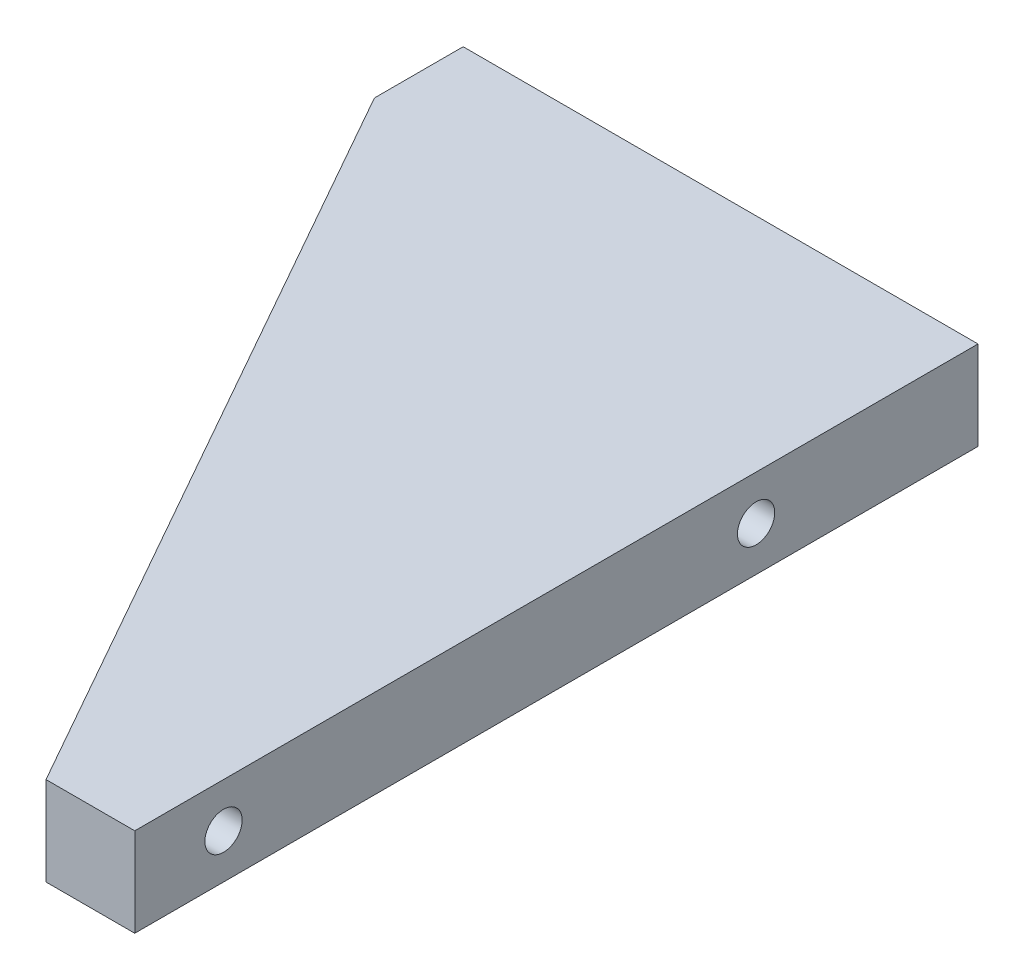
from build123d import *

# Parameters (mm, degrees)
SKETCH_1_W             = 58
SKETCH_1_H             = 95
EXTRUDE_1_DEPTH        = 5
CUT_EXTRUDE_1_DEPTH    = 10
HOLE_WIZARD_M5_1_D     = 4.2
HOLE_WIZARD_M5_1_DEPTH = 12.4
HOLE_WIZARD_M5_1_TIP   = 1.2618073
HOLE_WIZARD_M5_2_D     = 4.2
HOLE_WIZARD_M5_2_DEPTH = 12.4
HOLE_WIZARD_M5_2_TIP   = 1.2618073


with BuildPart() as part:
    # 草图1 → 凸台-拉伸1 (new, symmetric)
    with BuildSketch(Plane(origin=(0, 0, 0), x_dir=(1, 0, 0), z_dir=(0, 1, 0))):
        Rectangle(SKETCH_1_W, SKETCH_1_H)
    extrude(amount=EXTRUDE_1_DEPTH, both=True)

    # 草图2 → 切除-拉伸1 (cut)
    with BuildSketch(Plane(origin=(0, 5, 0), x_dir=(1, 0, 0), z_dir=(0, 1, 0))):
        Polygon((19, -47.5), (-29, 37.5), (-29, -47.5), align=None)
    extrude(amount=-CUT_EXTRUDE_1_DEPTH, mode=Mode.SUBTRACT)

    # M5 螺纹孔1
    with Locations(Plane(origin=(29, 0, 0), x_dir=(0, 0, -1), z_dir=(1, 0, 0))):
        with Locations((-37.5, 0), (22.5, 0)):
            Hole(HOLE_WIZARD_M5_1_D / 2, depth=HOLE_WIZARD_M5_1_DEPTH)
            with Locations((0, 0, -(HOLE_WIZARD_M5_1_DEPTH + HOLE_WIZARD_M5_1_TIP / 2))):  # 118° drill point
                Cone(0, HOLE_WIZARD_M5_1_D / 2, HOLE_WIZARD_M5_1_TIP, mode=Mode.SUBTRACT)

    # M5 螺纹孔2
    with Locations(Plane(origin=(0, 0, -47.5), x_dir=(-1, 0, 0), z_dir=(0, 0, -1))):
        with Locations((19, 0), (-21, 0)):
            Hole(HOLE_WIZARD_M5_2_D / 2, depth=HOLE_WIZARD_M5_2_DEPTH)
            with Locations((0, 0, -(HOLE_WIZARD_M5_2_DEPTH + HOLE_WIZARD_M5_2_TIP / 2))):  # 118° drill point
                Cone(0, HOLE_WIZARD_M5_2_D / 2, HOLE_WIZARD_M5_2_TIP, mode=Mode.SUBTRACT)


solid = part.part
